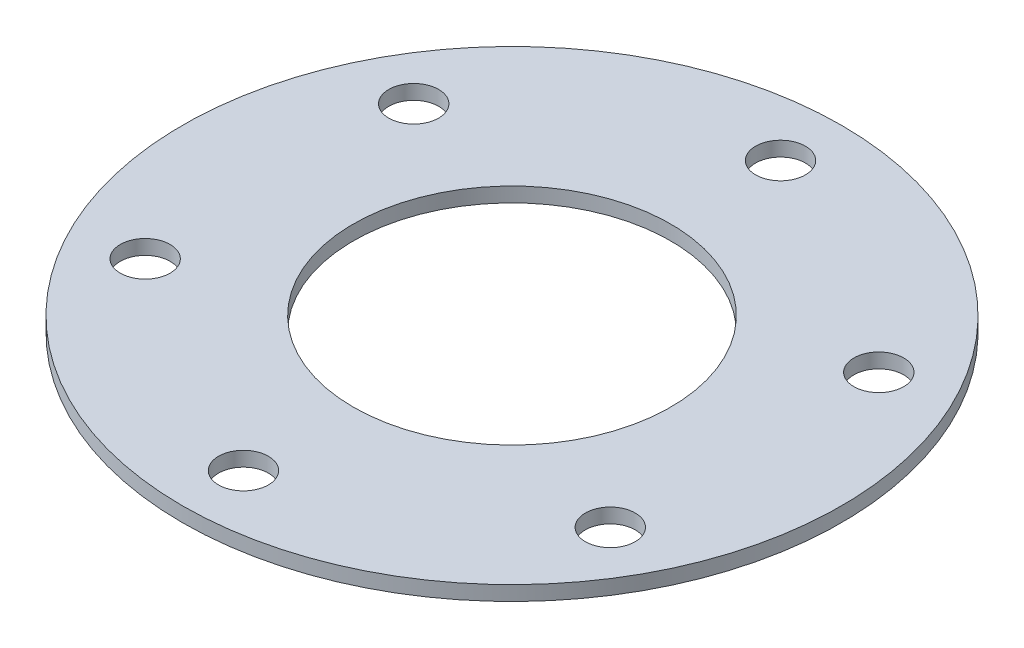
SolidWorks part; units mm, degrees
ref_plane "前视基准面" through (0, 0, 0) normal (0, 0, 1) x (1, 0, 0)
ref_plane "上视基准面" through (0, 0, 0) normal (0, 1, 0) x (1, 0, 0)
ref_plane "右视基准面" through (0, 0, 0) normal (1, 0, 0) x (0, 0, -1)
sketch "草图1" plane through (0, 0, 0) normal (0, 1, 0) x (1, 0, 0)
  circle A0 centre (0, 0) radius 67.5
  circle A1 centre (0, 0) radius 32.5
extrude "凸台-拉伸1" add sketch "草图1" along normal blind 3
hole_wizard "M12 螺纹孔的螺纹孔钻头1" positions "草图6" profile "草图5" hole size "M12" standard "Iso"
sketch "草图6" plane through (0, 3, 0) normal (0, 1, 0) x (1, 0, 0)
  line L2 (0, 0) -> (0, -50000) construction
  line L3 (0, 0) -> (43301.2702, 25000) construction
  line L4 (0, 0) -> (43301.2702, -25000) construction
  circle A0 centre (0, 0) radius 55 construction
  point P0 (0, 55)
  point P26 (-47.6314, 27.5)
  point P28 (-47.6314, -27.5)
  point P30 (0, -55)
  point P32 (47.6314, -27.5)
  point P34 (47.6314, 27.5)
  dimension "D1" = 60
  dimension "D2" = 60
sketch "草图5" plane through (0, 3, -55) normal (1, 0, 0) x (0, 0, 1)
  line L0 (0, 0) -> (0, 8.0644)
  line L1 (0, 8.0644) -> (5.1, 5)
  line L2 (5.1, 5) -> (5.1, 0)
  line L5 (5.1, 0) -> (0, 0)
  line L10 (0, 8.0644) -> (-5.1, 5) construction
  line L11 (0, -6.35) -> (0, 107.95) construction
  dimension "孔直径" = 10.2
  dimension "孔深度" = 5
  dimension "导头角度" = 118
